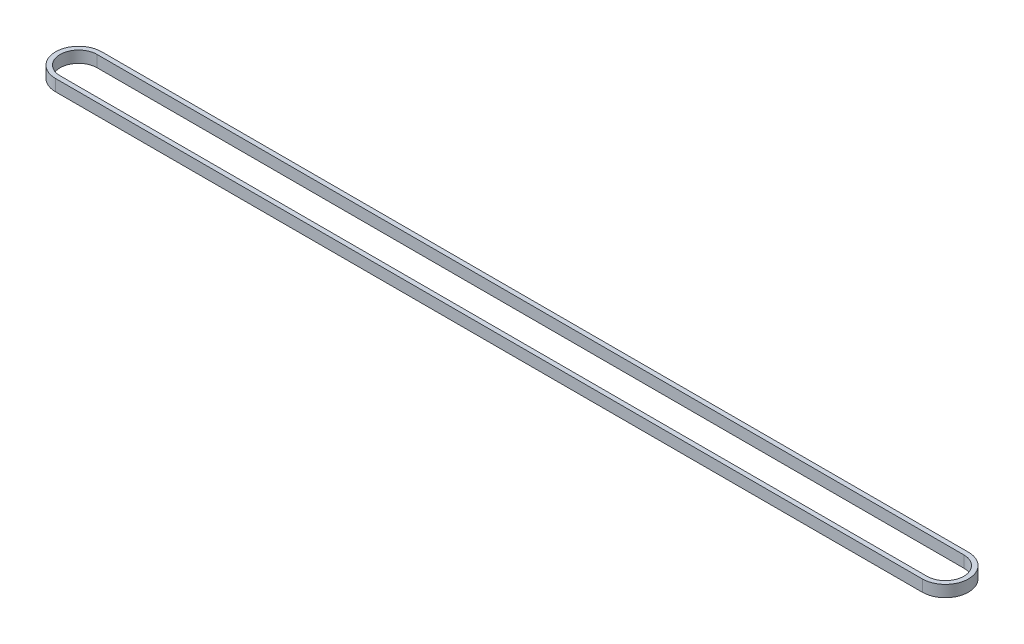
from build123d import *

# Parameters (mm, degrees)
BOSS_EXTRUDE1_DEPTH = 5


with BuildPart() as part:
    # Sketch1 → Boss-Extrude1 (new body)
    with BuildSketch(Plane(origin=(0, 0, 0), x_dir=(1, 0, 0), z_dir=(0, 1, 0))):
        with BuildLine():
            Line((-348.959440129, 10), (26.040559871, 10))
            ThreePointArc((26.040559871, 10), (36.040559871, 0), (26.040559871, -10))
            Line((26.040559871, -10), (-348.959440129, -10))
            ThreePointArc((-348.959440129, -10), (-358.959440129, 0), (-348.959440129, 10))
        make_face()
        with BuildLine():
            Line((-348.959440129, 8), (26.040559871, 8))
            ThreePointArc((26.040559871, 8), (34.040559871, 0), (26.040559871, -8))
            Line((26.040559871, -8), (-348.959440129, -8))
            ThreePointArc((-348.959440129, -8), (-356.959440129, 0), (-348.959440129, 8))
        make_face(mode=Mode.SUBTRACT)
    extrude(amount=BOSS_EXTRUDE1_DEPTH)


solid = part.part
